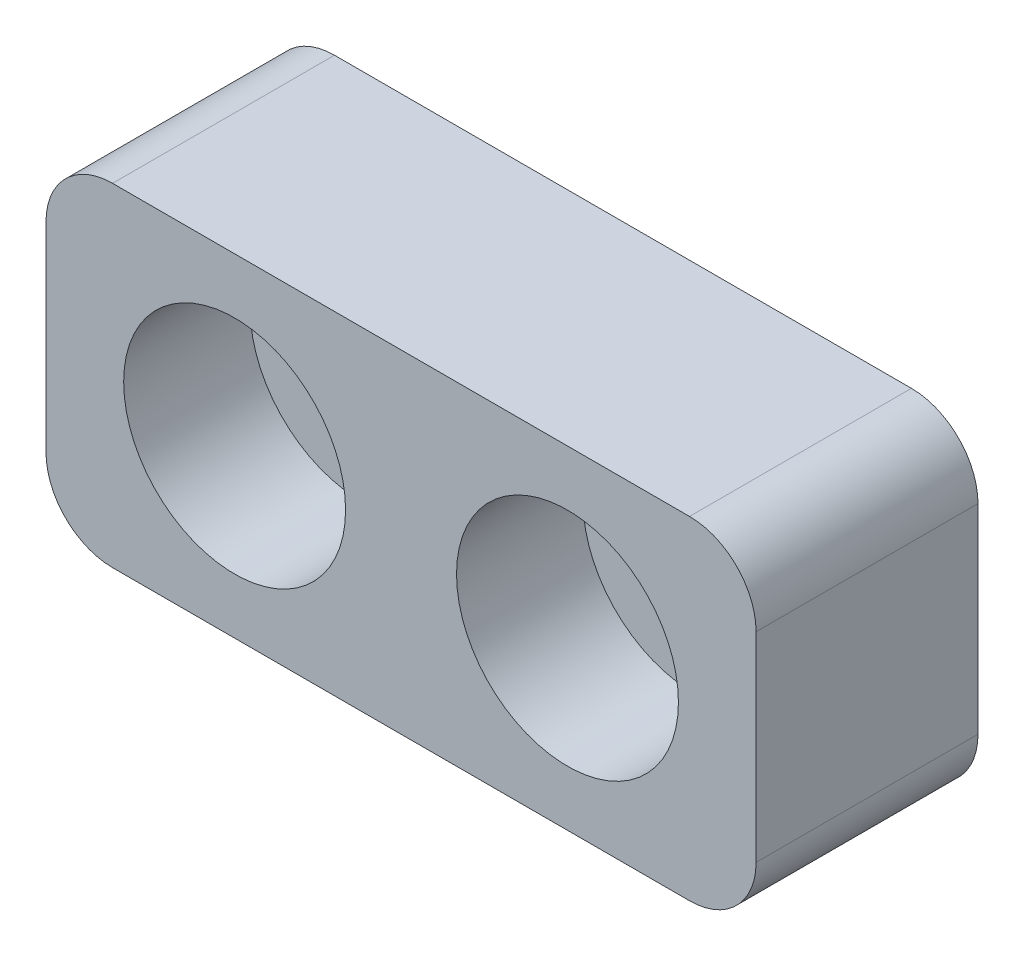
SolidWorks part; units mm, degrees
material "优力胶"
ref_plane "Front Plane" through (0, 0, 0) normal (0, 0, 1) x (1, 0, 0)
ref_plane "Top Plane" through (0, 0, 0) normal (0, 1, 0) x (1, 0, 0)
ref_plane "Right Plane" through (0, 0, 0) normal (1, 0, 0) x (0, 0, -1)
sketch "Sketch1" plane through (0, 0, 0) normal (0, 0, 1) x (1, 0, 0)
  line L1 (-16, -7.5) -> (16, -7.5)
  line L2 (-16, -7.5) -> (-16, 7.5)
  line L3 (-16, 7.5) -> (16, 7.5)
  line L4 (16, -7.5) -> (16, 7.5)
  line L5 (-16, -7.5) -> (16, 7.5) construction
  line L6 (-16, 7.5) -> (16, -7.5) construction
  point P0 (0, 0)
  dimension "D1" = 15
  dimension "D2" = 32
extrude "Boss-Extrude1" add sketch "Sketch1" along normal blind 10
hole_wizard "CBORE for M5 Hexagon socket head cap screws1" positions "Sketch2" profile "Sketch3" counterbore size "M5" standard "GB"
sketch "Sketch2" plane through (0, 0, 10) normal (0, 0, 1) x (1, 0, 0)
  line L0 (0, 7.5) -> (0, -7.5) construction
  line L1 (16, 7.5) -> (-16, 7.5) construction
  line L2 (-16, -7.5) -> (16, -7.5) construction
  line L4 (-16, 0) -> (16, 0) construction
  line L5 (-16, 7.5) -> (-16, -7.5) construction
  line L6 (16, -7.5) -> (16, 7.5) construction
  point P23 (-7.5, 0)
  point P25 (7.5, 0)
  dimension "D2" = 15
sketch "Sketch3" plane through (7.5, 0, 10) normal (1, 0, 0) x (0, -1, 0)
  line L0 (0, 0) -> (0, 14.0524)
  line L1 (0, 14.0524) -> (2.75, 12.4)
  line L2 (2.75, 12.4) -> (2.75, 5.7)
  line L3 (2.75, 5.7) -> (5, 5.7)
  line L4 (5, 5.7) -> (5, 0)
  line L5 (5, 0) -> (0, 0)
  line L10 (0, 14.0524) -> (-2.75, 12.4) construction
  line L11 (0, -6.35) -> (0, 107.95) construction
  dimension "孔直径" = 5.5
  dimension "孔深度" = 12.4
  dimension "柱形沉头孔直径" = 10
  dimension "柱形沉头孔深度" = 5.7
  dimension "导头角度" = 118
fillet "Fillet1" radius 3 4 edges at (16, -7.5, 5) (16, 7.5, 5) (-16, -7.5, 5) (-16, 7.5, 5)
